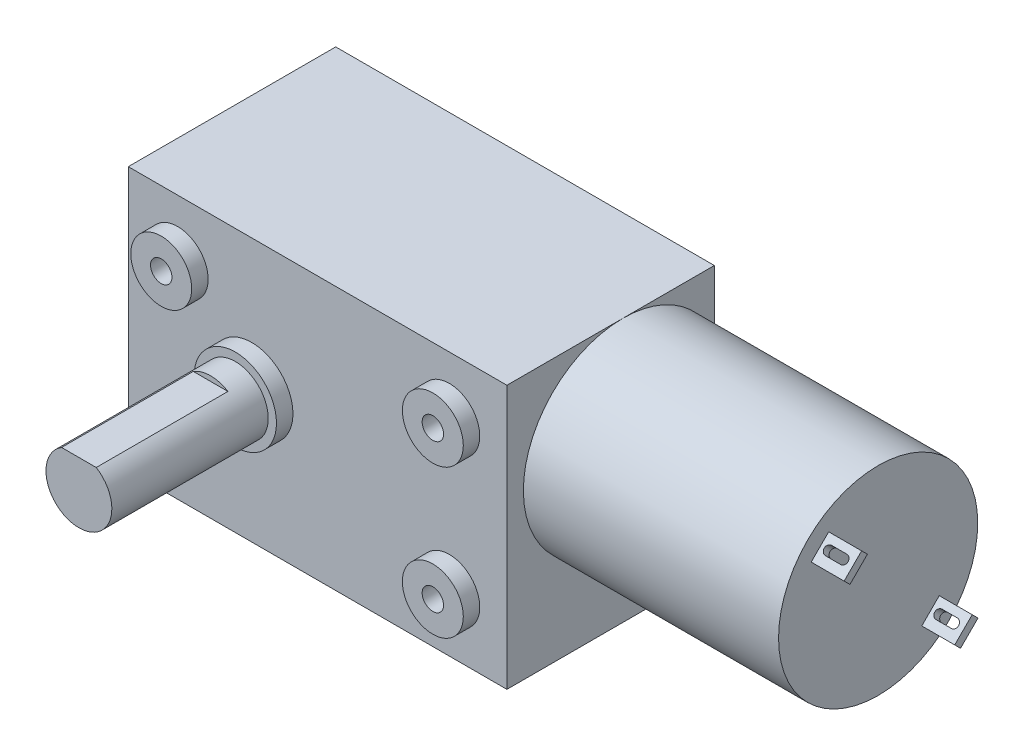
from build123d import *

# Parameters (mm, degrees)
SKETCH_1_W          = 46
SKETCH_1_H          = 32
EXTRUDE_1_DEPTH     = 25.2
SKETCH_2_R          = 3.7
SKETCH_2_R_2        = 5
EXTRUDE_2_DEPTH     = 2
SKETCH_3_R          = 1.3
CUT_EXTRUDE_1_DEPTH = 10
SKETCH_4_R          = 4
EXTRUDE_3_DEPTH     = 19
CUT_EXTRUDE_START   = -16
CUT_EXTRUDE_2_DEPTH = 16
SKETCH_6_R          = 12.1
EXTRUDE_4_DEPTH     = 31
EXTRUDE_5_DEPTH     = 4
CUT_EXTRUDE_3_DEPTH = 88.342884876


with BuildPart() as part:
    # 草图1 → 凸台-拉伸1 (new body)
    with BuildSketch(Plane.XY):
        with Locations((23, 16)):
            Rectangle(SKETCH_1_W, SKETCH_1_H)
    extrude(amount=EXTRUDE_1_DEPTH)

    # 草图2 → 凸台-拉伸2 (add)
    with BuildSketch(Plane.XY.offset(25.2)):
        with Locations(Location((6, 25, 0), (0, 0, 180))):
            Circle(SKETCH_2_R)
        with Locations(Location((6, 7, 0), (0, 0, 180))):
            Circle(SKETCH_2_R)
        with Locations(Location((39, 7, 0), (0, 0, 180))):
            Circle(SKETCH_2_R)
        with Locations(Location((39, 25, 0), (0, 0, 180))):
            Circle(SKETCH_2_R)
        with Locations(Location((15, 16, 0), (0, 0, 180))):
            Circle(SKETCH_2_R_2)
    extrude(amount=EXTRUDE_2_DEPTH)

    # 草图3 → 切除-拉伸1 (cut)
    with BuildSketch(Plane.XY.offset(27.2)):
        with Locations((6, 7)):
            Circle(SKETCH_3_R)
        with Locations((6, 25)):
            Circle(SKETCH_3_R)
        with Locations((39, 25)):
            Circle(SKETCH_3_R)
        with Locations((39, 7)):
            Circle(SKETCH_3_R)
    extrude(amount=-CUT_EXTRUDE_1_DEPTH, mode=Mode.SUBTRACT)

    # 草图4 → 凸台-拉伸3 (add)
    with BuildSketch(Plane.XY.offset(27.2)):
        with Locations((15, 16)):
            Circle(SKETCH_4_R)
    extrude(amount=EXTRUDE_3_DEPTH)

    # 草图5 → 切除-拉伸2 (cut)
    with BuildSketch(Plane.XY.offset(46.2).offset(CUT_EXTRUDE_START)):
        with BuildLine():
            Line((17.107130751, 19.4), (12.892869249, 19.4))
            ThreePointArc((12.892869249, 19.4), (15, 20), (17.107130751, 19.4))
        make_face()
    extrude(amount=CUT_EXTRUDE_2_DEPTH, mode=Mode.SUBTRACT)

    # 草图6 → 凸台-拉伸4 (add)
    with BuildSketch(Plane(origin=(46, 0, 0), x_dir=(0, 0, -1), z_dir=(1, 0, 0))):
        with Locations(Location((-11.1, 19.9, 0), (0, 0, 90))):
            Circle(SKETCH_6_R)
    extrude(amount=EXTRUDE_4_DEPTH)

    # 草图7 → 凸台-拉伸5 (add)
    with BuildSketch(Plane(origin=(77, 0, 0), x_dir=(0, 0, -1), z_dir=(1, 0, 0))):
        Polygon((-19.231728338, 25.910407286), (-17.110407994, 28.03172763), (-16.403301178, 27.324620884), (-18.524621557, 25.203300505), align=None)
        Polygon((-5.796699495, 12.475378443), (-3.675379152, 14.596698787), (-2.96827237, 13.889592006), (-5.089592714, 11.768271662), align=None)
    extrude(amount=EXTRUDE_5_DEPTH)

    # 草图8 → 切除-拉伸3 (cut, through all)
    with BuildSketch(Plane(origin=(0, 22.571067812, 22.571067812), x_dir=(1, 0, 0), z_dir=(0, 0.7071067811865464, 0.7071067811865487))):
        with BuildLine():
            Line((77.969259397, 6.842291957), (79.821949512, 6.842291957))
            ThreePointArc((79.821949512, 6.842291957), (80.341395338, 6.32284613), (79.821949512, 5.803400304))
            Line((79.821949512, 5.803400304), (77.969259397, 5.803400304))
            ThreePointArc((77.969259397, 5.803400304), (77.44981357, 6.32284613), (77.969259397, 6.842291957))
        make_face()
    extrude(amount=-CUT_EXTRUDE_3_DEPTH, mode=Mode.SUBTRACT)


solid = part.part
